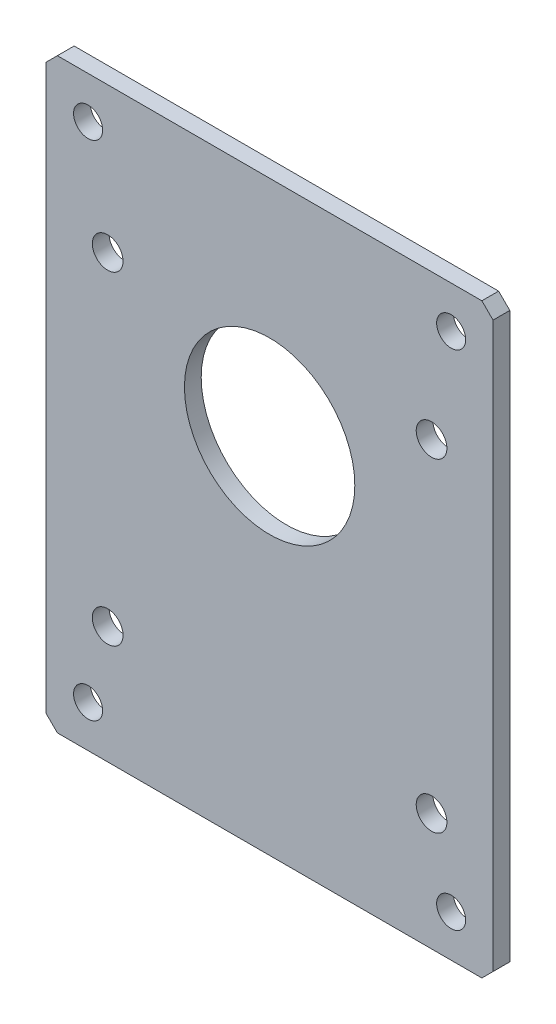
SolidWorks part; units mm, degrees
ref_plane "Front" through (0, 0, 0) normal (0, 0, 1) x (1, 0, 0)
ref_plane "Top" through (0, 0, 0) normal (0, 1, 0) x (1, 0, 0)
ref_plane "Right" through (0, 0, 0) normal (1, 0, 0) x (0, 0, -1)
sketch "Sketch1" plane through (0, 0, 0) normal (0, 0, 1) x (1, 0, 0)
  line L1 (0, 0) -> (80, 0)
  line L2 (0, 0) -> (0, 105)
  line L3 (0, 105) -> (80, 105)
  line L4 (80, 0) -> (80, 105)
  dimension "D1" = 80
  dimension "D2" = 105
extrude "Boss-Extrude1" add sketch "Sketch1" along normal blind 3
sketch "Sketch2" plane through (0, 0, 3) normal (0, 0, 1) x (1, 0, 0)
  line L0 (40, 105) -> (40, 0) construction
  line L1 (80, 105) -> (0, 105) construction
  line L2 (0, 0) -> (80, 0) construction
  line L3 (0, 52.5) -> (80, 52.5) construction
  line L4 (0, 105) -> (0, 0) construction
  line L5 (80, 0) -> (80, 105) construction
  circle A0 centre (7.5, 97.5) radius 2.6
  circle A1 centre (72.5, 97.5) radius 2.6
  circle A2 centre (7.5, 7.5) radius 2.6
  circle A3 centre (72.5, 7.5) radius 2.6
  circle A4 centre (40, 65) radius 15.25
  dimension "D1" = 5.2
  dimension "D2" = 65
  dimension "D3" = 90
  dimension "D4" = 30.5
  dimension "D5" = 40
extrude "Cut-Extrude1" cut sketch "Sketch2" against normal blind 10
hole_wizard "M5 Tapped Hole1" positions "Sketch5" profile "Sketch4" tap size "M5" standard "GB"
sketch "Sketch5" plane through (0, 0, 3) normal (0, 0, 1) x (1, 0, 0)
  line L0 (0, 50) -> (80, 50) construction
  line L5 (40, 50) -> (11.0086, 78.9914) construction
  line L8 (40, 50) -> (68.9914, 78.9914) construction
  line L11 (40, 50) -> (40, 91) construction
  line L14 (80, 105) -> (0, 105) construction
  circle A0 centre (40, 50) radius 41 construction
  circle A2 centre (40, 65) radius 15.25 construction
  point P0 (11.0086, 78.9914)
  point P1 (68.9914, 78.9914)
  point P3 (11.0086, 21.0086)
  point P5 (68.9914, 21.0086)
  point P44 (40, 105)
  dimension "D1" = 82
  dimension "D4" = 15
  dimension "D2" = 45
  dimension "D3" = 45
sketch "Sketch4" plane through (11.0086, 78.9914, 3) normal (1, 0, 0) x (0, -1, 0)
  line L0 (0, 0) -> (0, 13.6618)
  line L1 (0, 13.6618) -> (2.1, 12.4)
  line L2 (2.1, 12.4) -> (2.1, 0)
  line L5 (2.1, 0) -> (0, 0)
  line L10 (0, 13.6618) -> (-2.1, 12.4) construction
  line L11 (0, -6.35) -> (0, 107.95) construction
  dimension "螺纹孔钻头直径" = 4.2
  dimension "螺纹孔钻头深度" = 12.4
  dimension "导头角度" = 118
cosmetic thread "Cosmetic Thread1" parameters "D1"=10, "D2"=5
cosmetic thread "Cosmetic Thread2" parameters "D1"=10, "D2"=5
cosmetic thread "Cosmetic Thread3" parameters "D1"=10, "D2"=5
cosmetic thread "Cosmetic Thread4" parameters "D1"=10, "D2"=5
chamfer "Chamfer1" distance 2 angle 45 4 edges at (0, 0, 1.5) (80, 0, 1.5) (0, 105, 1.5) (80, 105, 1.5)
sketch "Sketch6" plane through (0, 0, 0) normal (0, 0, -1) x (-1, 0, 0)
  circle A0 centre (-68.9914, 78.9914) radius 2.75
  circle A1 centre (-11.0086, 78.9914) radius 2.75
  circle A2 centre (-68.9914, 21.0086) radius 2.75
  circle A3 centre (-11.0086, 21.0086) radius 2.75
  dimension "D1" = 5.5
extrude "Cut-Extrude3" cut sketch "Sketch6" against normal through all
